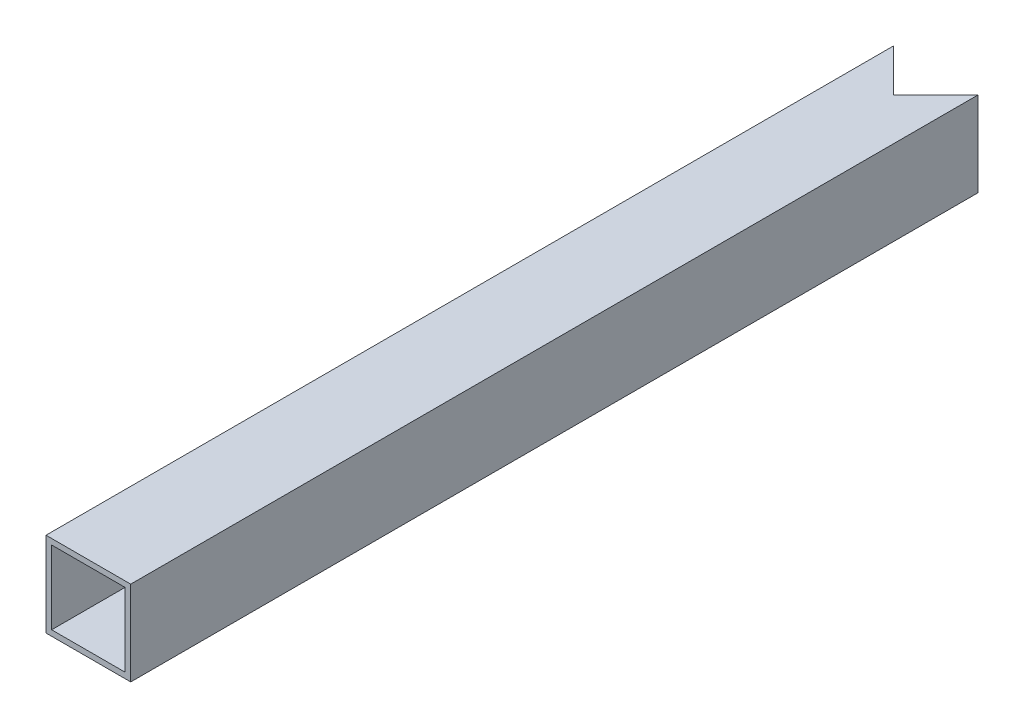
SolidWorks part; units mm, degrees
ref_plane "前视基准面" through (0, 0, 0) normal (0, 0, 1) x (1, 0, 0)
ref_plane "上视基准面" through (0, 0, 0) normal (0, 1, 0) x (1, 0, 0)
ref_plane "右视基准面" through (0, 0, 0) normal (1, 0, 0) x (0, 0, -1)
sketch "草图1" plane through (0, 0, 0) normal (0, 0, 1) x (1, 0, 0)
  line L0 (13, -13) -> (13, 13)
  line L1 (15, -15) -> (-15, -15)
  line L2 (15, -15) -> (15, 15)
  line L3 (15, 15) -> (-15, 15)
  line L4 (-15, -15) -> (-15, 15)
  line L5 (15, -15) -> (-15, 15) construction
  line L6 (15, 15) -> (-15, -15) construction
  line L7 (13, 13) -> (-13, 13)
  line L8 (-13, -13) -> (-13, 13)
  line L9 (13, -13) -> (-13, -13)
  point P0 (0, 0)
  dimension "D1" = 30
  dimension "D2" = 2
extrude "凸台-拉伸1" add sketch "草图1" along normal mid plane 300
sketch "草图2" plane through (0, 0, 150) normal (0, 0, 1) x (1, 0, 0)
  circle A1 centre (0, 0) radius 4.2683
sketch "草图3" plane through (0, 15, 0) normal (0, 1, 0) x (1, 0, 0)
  line L0 (-15, 150) -> (0, 135)
  line L1 (0, 135) -> (15, 150)
  line L6 (15, 150) -> (-15, 150)
  line L7 (-15, 150) -> (-15, -150)
  line L8 (-15, -150) -> (15, -150)
  line L9 (15, -150) -> (15, 150)
  line L10 (15, 150) -> (-15, 150)
  dimension "D1" = 0
extrude "切除-拉伸1" cut sketch "草图3" against normal blind 102
